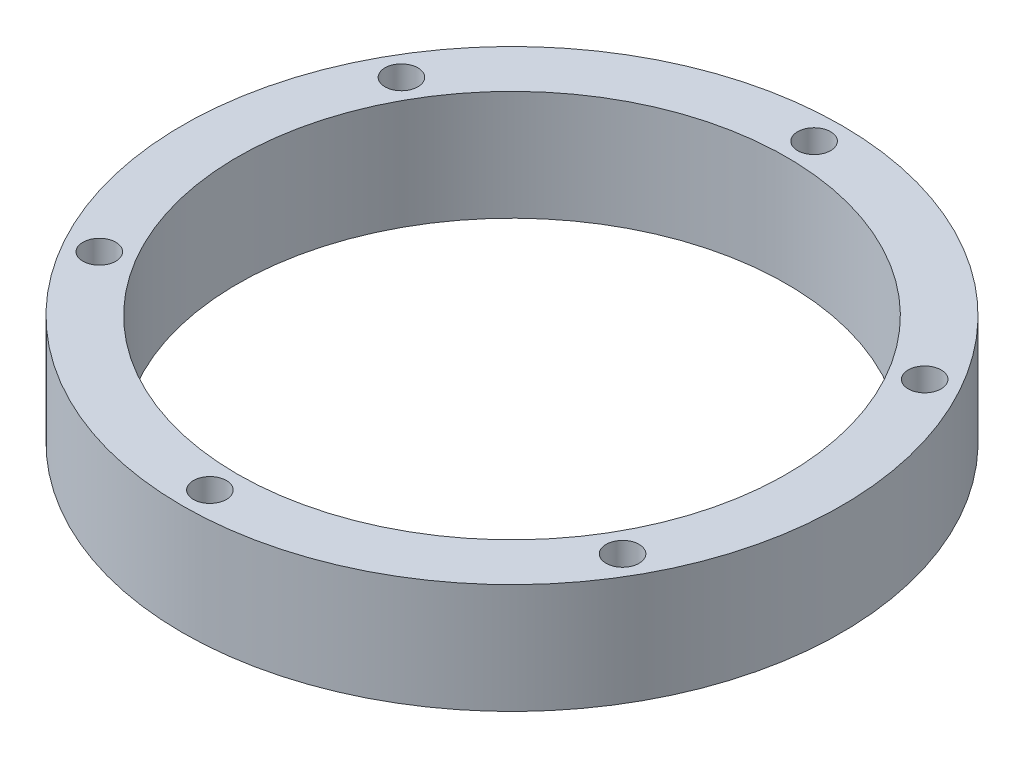
SolidWorks part; units mm, degrees
ref_plane "前视基准面" through (0, 0, 0) normal (0, 0, 1) x (1, 0, 0)
ref_plane "上视基准面" through (0, 0, 0) normal (0, 1, 0) x (1, 0, 0)
ref_plane "右视基准面" through (0, 0, 0) normal (1, 0, 0) x (0, 0, -1)
sketch "草图1" plane through (0, 0, 0) normal (0, 1, 0) x (1, 0, 0)
  circle A0 centre (0, 0) radius 50
  circle A1 centre (0, 0) radius 60
  dimension "D1" = 120
  dimension "D2" = 100
extrude "凸台-拉伸1" add sketch "草图1" along normal blind 20
sketch "草图2" plane through (0, 20, 0) normal (0, 1, 0) x (1, 0, 0)
  circle A0 centre (0, 55) radius 3
  dimension "D1" = 55
extrude "切除-拉伸1" cut sketch "草图2" against normal through all
pattern_circular "阵列(圆周)1" count 6 over 360 about axis through (0, 0, 0) along (0, 1, 0) of "切除-拉伸1"
